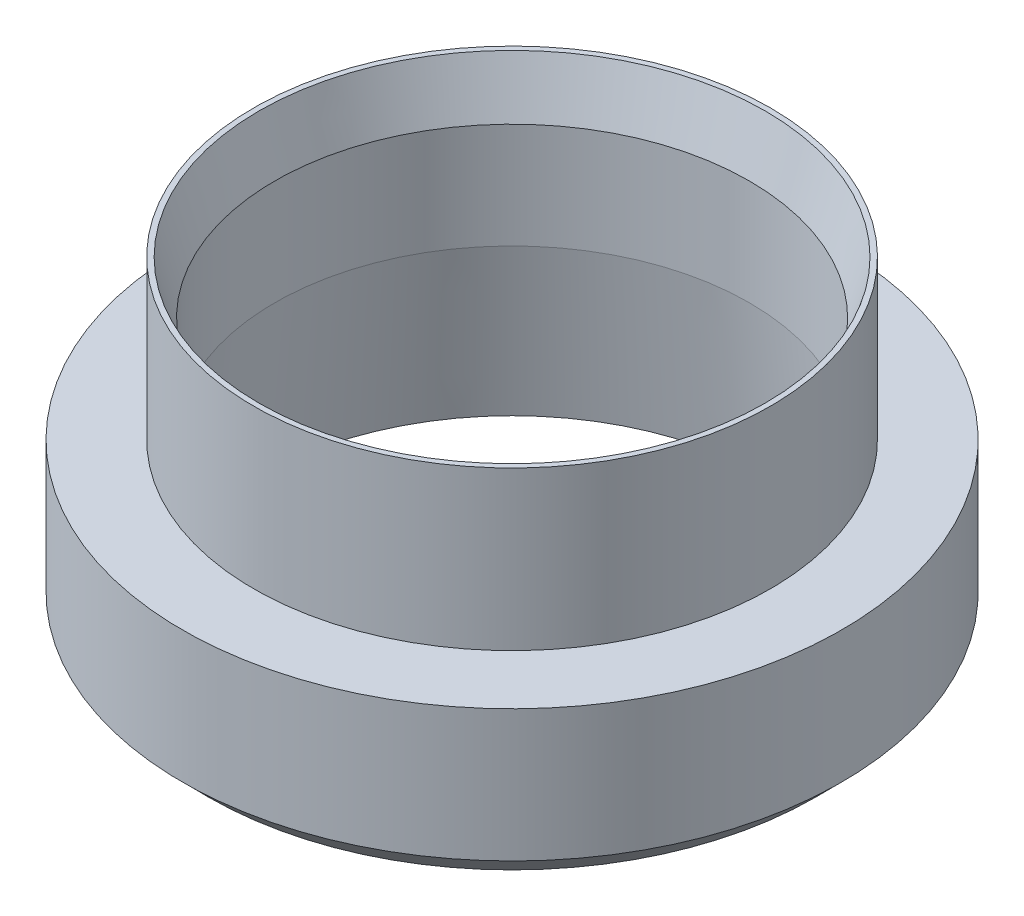
SolidWorks part; units mm, degrees
ref_plane "Front Plane" through (0, 0, 0) normal (0, 0, 1) x (1, 0, 0)
ref_plane "Top Plane" through (0, 0, 0) normal (0, 1, 0) x (1, 0, 0)
ref_plane "Right Plane" through (0, 0, 0) normal (1, 0, 0) x (0, 0, -1)
sketch "Sketch2" plane through (0, 0, 0) normal (0, 0, 1) x (1, 0, 0)
  line L0 (4.5, 0) -> (4.5, 6)
  line L1 (4.5, 6) -> (4.9, 6)
  line L2 (4.9, 6) -> (4.9, 3)
  line L3 (4.9, 3) -> (6.25, 3)
  line L4 (6.25, 3) -> (6.25, 0)
  line L5 (6.25, 0) -> (4.5, 0)
  line L6 (0, 0) -> (0, 26.7053) construction
  dimension "D1" = 4.5
  dimension "D2" = 1.75
  dimension "D3" = 3
  dimension "D5" = 0.4
  dimension "D6" = 6
revolve "Revolve1" add sketch "Sketch2" angle 360 about L6
sketch "Sketch3" plane through (0, 0, 0) normal (0, 0, 1) x (1, 0, 0)
  line L0 (4.5, 3) -> (4.5, 0)
  line L1 (4.5, 0) -> (4.8, 0)
  line L2 (4.8, 0) -> (4.5, 3)
  line L3 (-6.25, 0) -> (6.25, 0) construction
  line L4 (4.5, 0) -> (4.5, 6) construction
  line L5 (0, 0) -> (0, 3.714) construction
  dimension "D1" = 0.3
  dimension "D2" = 3
revolve "Cut-Revolve1" cut sketch "Sketch3" angle 360 about L5
chamfer "Chamfer1" distance 0.5 angle 45 1 edges at (0, 0, -6.25)
chamfer "Chamfer2" distance 1 distance2 0.3 1 edges at (0, 6, -4.5)
